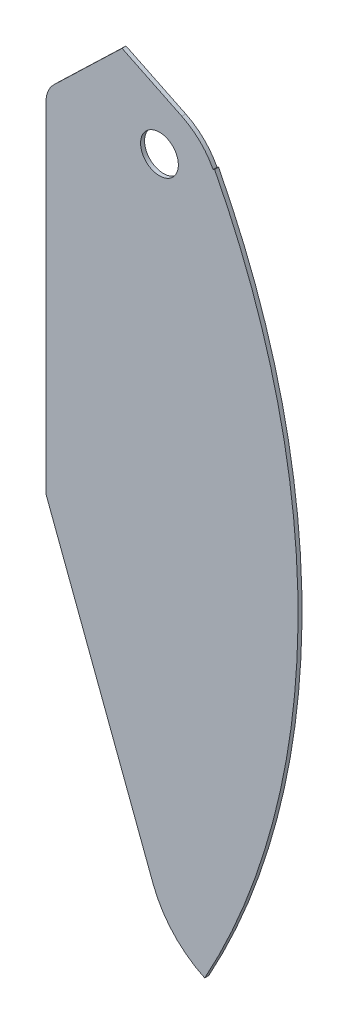
from build123d import *

# Parameters (mm, degrees)
SKETCH1_R           = 38.1
BOSS_EXTRUDE1_DEPTH = 4


with BuildPart() as part:
    # Sketch1 → Boss-Extrude1 (new, symmetric)
    with BuildSketch(Plane.XY):
        with BuildLine():
            Line((1000.125, 641.35), (1000.125, -45.0629))
            Line((1000.125, -45.0629), (1215.934413963, -617.113829271))
            ThreePointArc((1215.934413963, -617.113829271), (1256.96824156, -683.459757951), (1319.975225131, -729.45625))
            ThreePointArc((1319.975225131, -729.45625), (1507.976686944, -21.150112495), (1339.913949896, 692.15))
            Line((1339.913949896, 692.15), (1336.870808151, 690.572164727))
            ThreePointArc((1336.870808151, 690.572164727), (1310.307279769, 726.359551875), (1273.824497124, 751.959643467))
            Line((1273.824497124, 751.959643467), (1153.31875, 810.41875))
            Line((1153.31875, 810.41875), (1015.69584463, 677.949817102))
            ThreePointArc((1015.69584463, 677.949817102), (1004.179513091, 661.237168064), (1000.125, 641.35))
        make_face()
        with Locations((1228.725, 663.575)):
            Circle(SKETCH1_R, mode=Mode.SUBTRACT)
    extrude(amount=BOSS_EXTRUDE1_DEPTH, both=True)


solid = part.part
